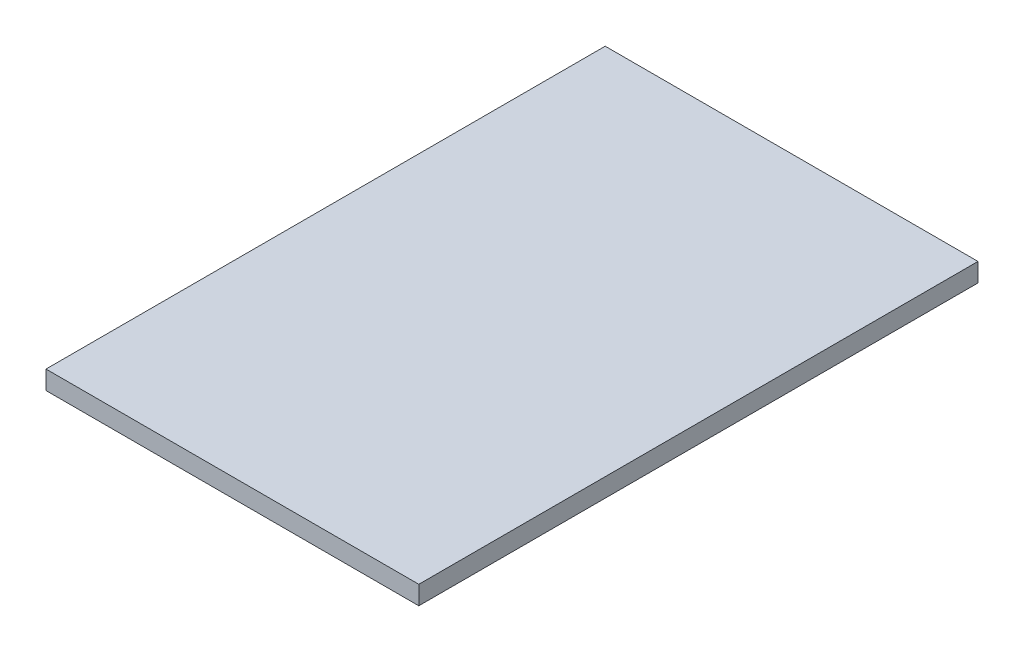
from build123d import *

# Parameters (mm, degrees)
SKETCH1_W           = 200
SKETCH1_H           = 300
BOSS_EXTRUDE1_DEPTH = 10


with BuildPart() as part:
    # Sketch1 → Boss-Extrude1 (new body)
    with BuildSketch(Plane(origin=(0, 0, 0), x_dir=(1, 0, 0), z_dir=(0, 1, 0))):
        Rectangle(SKETCH1_W, SKETCH1_H)
    extrude(amount=BOSS_EXTRUDE1_DEPTH)


solid = part.part
